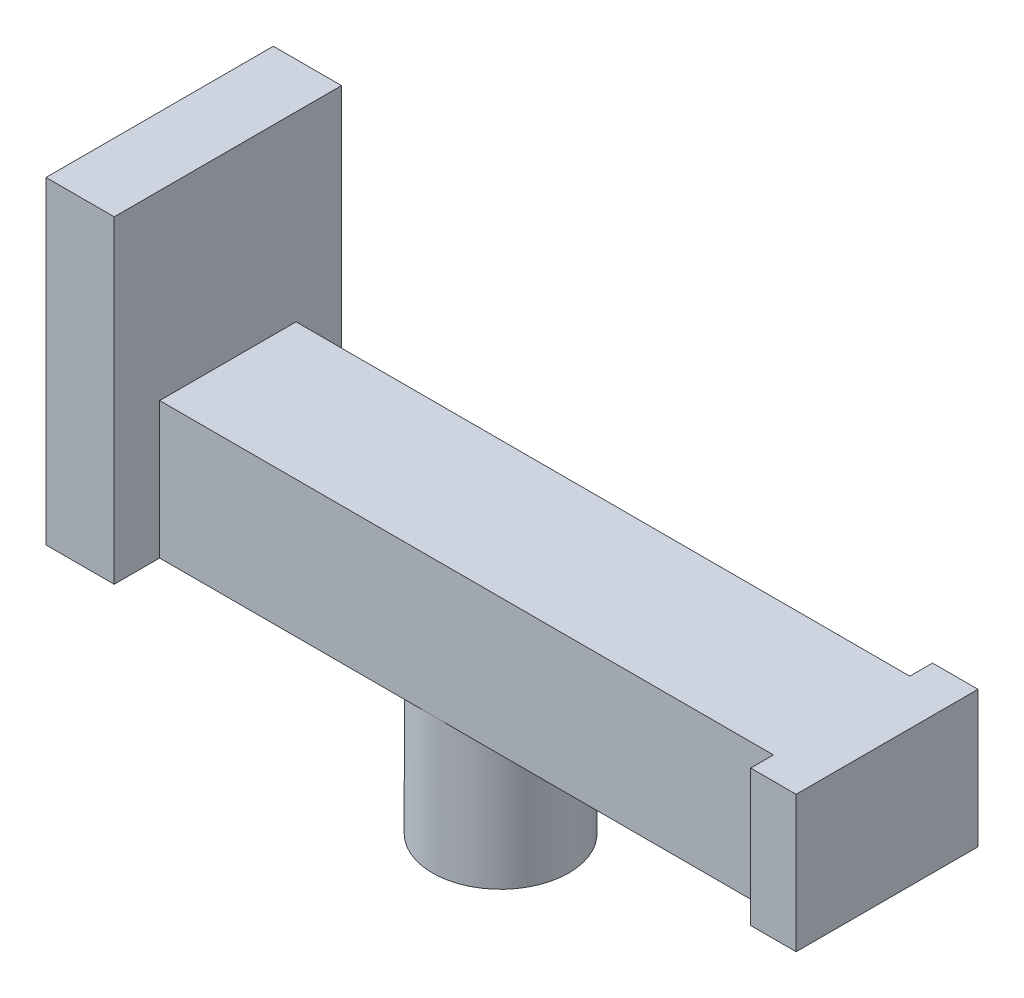
SolidWorks part; units mm, degrees
ref_plane "Front Plane" through (0, 0, 0) normal (0, 0, 1) x (1, 0, 0)
ref_plane "Top Plane" through (0, 0, 0) normal (0, 1, 0) x (1, 0, 0)
ref_plane "Right Plane" through (0, 0, 0) normal (1, 0, 0) x (0, 0, -1)
sketch "Sketch1" plane through (0, 0, 0) normal (0, 0, 1) x (1, 0, 0)
  line L1 (25, -3) -> (-25, -3)
  line L2 (25, -3) -> (25, 3)
  line L3 (25, 3) -> (-25, 3)
  line L4 (-25, -3) -> (-25, 3)
  line L5 (25, -3) -> (-25, 3) construction
  line L6 (25, 3) -> (-25, -3) construction
  point P0 (0, 0)
  dimension "D1" = 50
  dimension "D2" = 6
extrude "Boss-Extrude1" add sketch "Sketch1" along normal blind 6
sketch "Sketch2" plane through (0, -3, 0) normal (0, -1, 0) x (1, 0, 0)
  line L0 (-25, 6) -> (-25, 0) construction
  circle A0 centre (-10, 3) radius 3
  dimension "D2" = 6
  dimension "D1" = 15
extrude "Boss-Extrude2" add sketch "Sketch2" along normal blind 6
sketch "Sketch3" plane through (-25, 0, 0) normal (-1, 0, 0) x (0, 0, 1)
  line L0 (3, -9) -> (3, 3) construction
  line L1 (-2, 3) -> (8, 3)
  line L2 (-2, 3) -> (-2, -3)
  line L3 (-2, -3) -> (8, -3)
  line L4 (8, 3) -> (8, -3)
  line L5 (-2, 3) -> (8, -3) construction
  line L6 (-2, -3) -> (8, 3) construction
  line L7 (0, -9) -> (6, -9) construction
  point P0 (3, 0)
  dimension "D1" = 10
extrude "Boss-Extrude3" add sketch "Sketch3" against normal blind 3
sketch "Sketch4" plane through (25, 0, 0) normal (1, 0, 0) x (0, 0, -1)
  line L8 (0, -3) -> (0, 3)
  line L9 (0, 3) -> (-6, 3)
  line L10 (-6, 3) -> (-6, -3)
  line L11 (-6, -3) -> (0, -3)
  line L12 (0, -3) -> (0, 3)
  line L13 (0, 3) -> (-6, 3)
  line L14 (-6, 3) -> (-6, -3)
  line L15 (-6, -3) -> (0, -3)
  dimension "D1" = 0
extrude "Cut-Extrude1" cut sketch "Sketch4" against normal blind 20
sketch "Sketch5" plane through (5, 0, 0) normal (1, 0, 0) x (0, 0, -1)
  line L0 (2, -3) -> (0, -3) construction
  line L1 (-7, 3) -> (1, 3)
  line L2 (-7, 3) -> (-7, -3)
  line L3 (-7, -3) -> (1, -3)
  line L4 (1, 3) -> (1, -3)
  line L5 (-7, 3) -> (1, -3) construction
  line L6 (-7, -3) -> (1, 3) construction
  point P0 (-3, 0)
  dimension "D1" = 8
extrude "Boss-Extrude4" add sketch "Sketch5" along normal blind 2
sketch "Sketch6" plane through (0, 3, 0) normal (0, 1, 0) x (1, 0, 0)
  line L1 (-25, 2) -> (-22, 2)
  line L2 (-25, 2) -> (-25, -8)
  line L3 (-25, -8) -> (-22, -8)
  line L4 (-22, 2) -> (-22, -8)
extrude "Boss-Extrude5" add sketch "Sketch6" along normal blind 8
